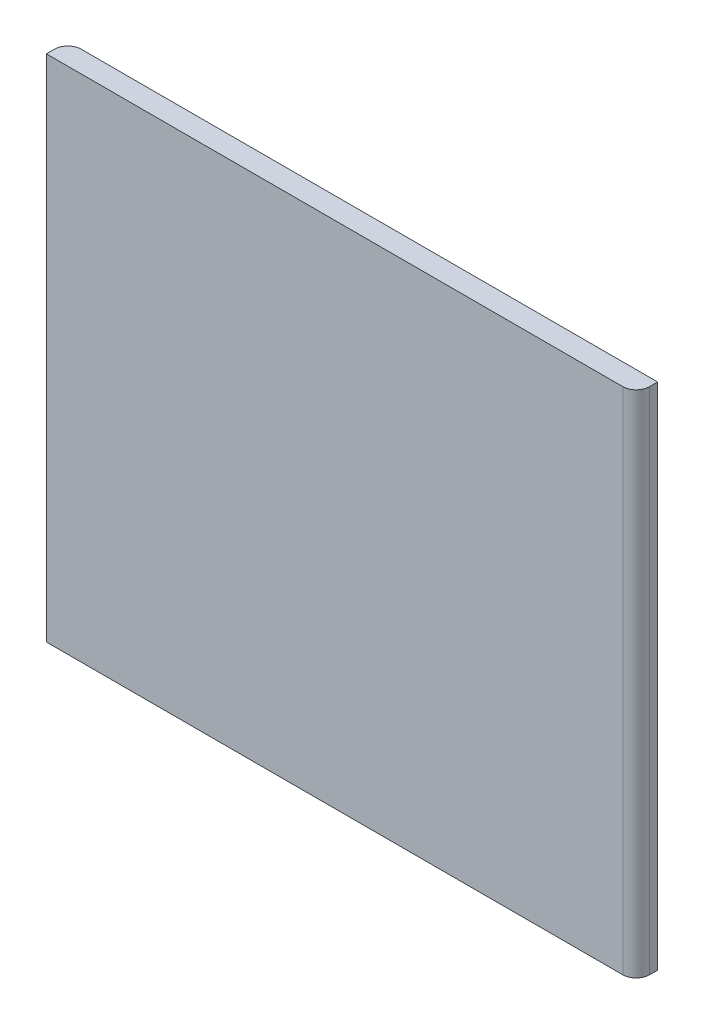
SolidWorks part; units mm, degrees
material "1023 Carbon steel plate (SS)"
ref_plane "Front Plane" through (0, 0, 0) normal (0, 0, 1) x (1, 0, 0)
ref_plane "Top Plane" through (0, 0, 0) normal (0, 1, 0) x (1, 0, 0)
ref_plane "Right Plane" through (0, 0, 0) normal (1, 0, 0) x (0, 0, -1)
sketch "Sketch1" plane through (0, 0, 0) normal (0, 0, 1) x (1, 0, 0)
  line L1 (-110, 95) -> (110, 95)
  line L2 (-110, 95) -> (-110, -95)
  line L3 (-110, -95) -> (110, -95)
  line L4 (110, 95) -> (110, -95)
  line L5 (-110, 95) -> (110, -95) construction
  line L6 (-110, -95) -> (110, 95) construction
  point P0 (0, 0)
  dimension "D1" = 190
  dimension "D2" = 220
extrude "Boss-Extrude1" add sketch "Sketch1" along normal blind 8
fillet "Fillet1" radius 5 2 edges at (110, 0, 8) (-110, 0, 0)
